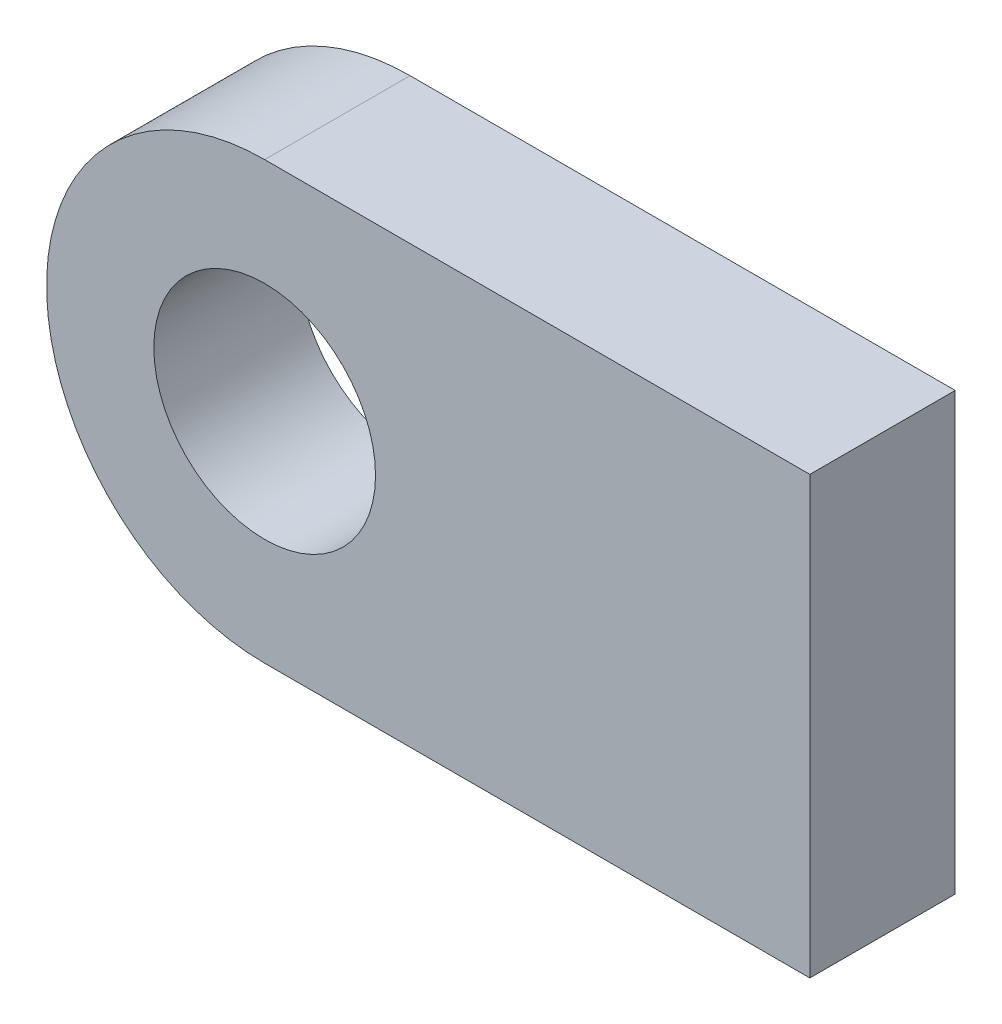
SolidWorks part; units mm, degrees
ref_plane "前视基准面" through (0, 0, 0) normal (0, 0, 1) x (1, 0, 0)
ref_plane "上视基准面" through (0, 0, 0) normal (0, 1, 0) x (1, 0, 0)
ref_plane "右视基准面" through (0, 0, 0) normal (1, 0, 0) x (0, 0, -1)
other "Configuration Table"
sketch "草图1" plane through (0, 0, 0) normal (0, 0, 1) x (1, 0, 0)
  line L0 (0, 12) -> (30, 12)
  line L1 (30, 12) -> (30, -12)
  line L2 (30, -12) -> (0, -12)
  arc A0 (0, -12) -> (0, 12) centre (0, 0) cw
  circle A1 centre (0, 0) radius 6.1
  point P0 (0, 0)
  dimension "D1" = 12.2
  dimension "D2" = 12
  dimension "D3" = 30
extrude "凸台-拉伸1" add sketch "草图1" against normal mid plane 8
